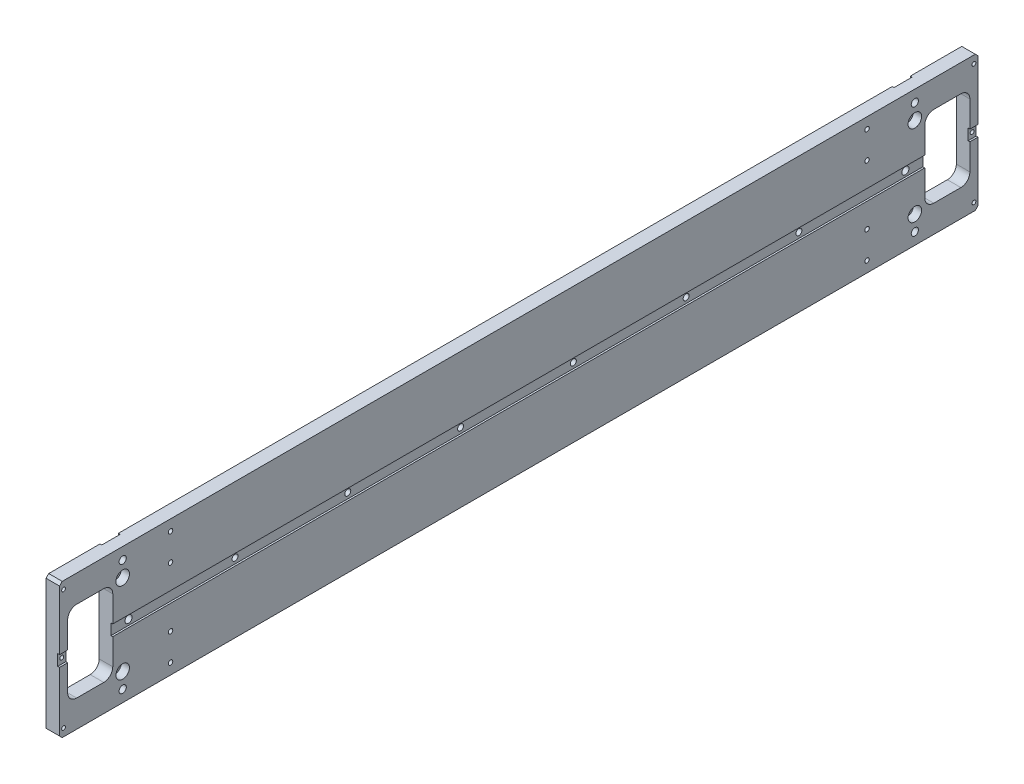
from build123d import *

# Parameters (mm, degrees)
SKETCH_1_W                  = 1018
SKETCH_1_H                  = 150
EXTRUDE_1_DEPTH             = 15
SKETCH_2_W                  = 1412.201465812
SKETCH_2_H                  = 12.2
CUT_EXTRUDE_1_DEPTH         = 2
SKETCH_15_W                 = 20.2
SKETCH_15_H                 = 532.053707348
SKETCH_15_H_2               = 612.26589084
CUT_EXTRUDE_4_DEPTH         = 2
CHAMFER_1_SIZE              = 3
SKETCH_24_W                 = 50
SKETCH_24_H                 = 90
CUT_EXTRUDE_5_DEPTH         = 515.714483962
FILLET_2_R                  = 10
FILLET_2_OF_MIRROR_1_R      = 10
HOLE_WIZARD_9_D             = 9
HOLE_WIZARD_9_CBORE_D       = 15
HOLE_WIZARD_9_CBORE_DEPTH   = 9
MM_2_AT_2_COUNT             = 2
MM_2_AT_2_PITCH             = 124
HOLE_WIZARD_M6_1_D          = 5
HOLE_WIZARD_9_2_D           = 6.6
HOLE_WIZARD_9_2_CBORE_D     = 11
HOLE_WIZARD_9_2_CBORE_DEPTH = 6.8
MM_3_D                      = 8
HOLE_WIZARD_0_D             = 4.3
HOLE_WIZARD_0_CBORE_D       = 8
HOLE_WIZARD_0_CBORE_DEPTH   = 5


with BuildPart() as part:
    # 草图1 → 凸台-拉伸1 (new body)
    with BuildSketch(Plane(origin=(0, 0, 0), x_dir=(0, 0, -1), z_dir=(1, 0, 0))):
        Rectangle(SKETCH_1_W, SKETCH_1_H)
    extrude(amount=EXTRUDE_1_DEPTH)

    # 草图2 → 切除-拉伸1 (cut)
    with BuildSketch(Plane(origin=(15, 0, 0), x_dir=(0, 0, -1), z_dir=(1, 0, 0))):
        Rectangle(SKETCH_2_W, SKETCH_2_H)
    extrude(amount=-CUT_EXTRUDE_1_DEPTH, mode=Mode.SUBTRACT)

    # 草图15 → 切除-拉伸4 (cut)
    with BuildSketch(Plane.ZY):
        with Locations((-439, -14.180103386)):
            Rectangle(SKETCH_15_W, SKETCH_15_H)
        with Locations((439, -22.190357802)):
            Rectangle(SKETCH_15_W, SKETCH_15_H_2)
    extrude(amount=-CUT_EXTRUDE_4_DEPTH, mode=Mode.SUBTRACT)

    # 倒角1
    chamfer_1_edges = [part.edges().sort_by_distance(p)[0] for p in [
        (7.5, 75, 509),
        (7.5, 75, -509),
        (7.5, -75, -509),
        (7.5, -75, 509),
    ]]
    chamfer(chamfer_1_edges, length=CHAMFER_1_SIZE)

    # 草图24 → 切除-拉伸5 (cut, through all)
    with BuildSketch(Plane(origin=(15, 0, 0), x_dir=(0, 0, -1), z_dir=(1, 0, 0))):
        with Locations((-475, 0)):
            Rectangle(SKETCH_24_W, SKETCH_24_H)
    cut_extrude_5 = extrude(amount=-CUT_EXTRUDE_5_DEPTH, mode=Mode.SUBTRACT)

    # 圆角2
    fillet_2_edges = [part.edges().sort_by_distance(p)[0] for p in [
        (7.5, 45, 450),
        (7.5, -45, 500),
        (7.5, -45, 450),
        (7.5, 45, 500),
    ]]
    fillet(fillet_2_edges, radius=FILLET_2_R)

    # 镜向1: 切除-拉伸5 across plane
    add(cut_extrude_5.mirror(Plane.XY), mode=Mode.SUBTRACT)

    # 圆角2 of 镜向1
    fillet_2_of_mirror_1_edges = [part.edges().sort_by_distance(p)[0] for p in [
        (7.5, 45, -450),
        (7.5, -45, -500),
        (7.5, -45, -450),
        (7.5, 45, -500),
    ]]
    fillet(fillet_2_of_mirror_1_edges, radius=FILLET_2_OF_MIRROR_1_R)

    # Hole Wizard 9 (through all)
    with Locations(Plane(origin=(15, 0, 0), x_dir=(0, 0, -1), z_dir=(1, 0, 0))):
        with Locations((439, 45), (439, -45)):
            hole_wizard_9 = CounterBoreHole(HOLE_WIZARD_9_D / 2, HOLE_WIZARD_9_CBORE_D / 2, HOLE_WIZARD_9_CBORE_DEPTH)

    # 草图34 → 大小mm 暗销孔2 (revolve, cut)
    with BuildSketch(Plane(origin=(15, 62, -439), x_dir=(0, 0, -1), z_dir=(0, 1, 0))):
        Polygon((0, 0), (0, 17.403442476), (4, 15), (4, 0), align=None)
    mm_2 = revolve(axis=Axis((21.35, 62, -439), (-1, 0, 0)), mode=Mode.SUBTRACT)

    # 大小mm 暗销孔2 at 2: 大小mm 暗销孔2 ×2
    with Locations(*[(0, -i * MM_2_AT_2_PITCH, 0) for i in range(1, MM_2_AT_2_COUNT)]):
        add(mm_2, mode=Mode.SUBTRACT)

    # M6 螺纹孔1 (through all)
    with Locations(Plane.ZY):
        with Locations((-386, 63), (-386, 33), (-386, -33), (-386, -63)):
            hole_wizard_m6_1 = Hole(HOLE_WIZARD_M6_1_D / 2)

    # Hole Wizard 9 2 (through all)
    with Locations(Plane.ZY):
        with Locations((-312.5, 0), (-187.5, 0), (-62.5, 0), (62.5, 0), (187.5, 0), (312.5, 0)):
            CounterBoreHole(HOLE_WIZARD_9_2_D / 2, HOLE_WIZARD_9_2_CBORE_D / 2, HOLE_WIZARD_9_2_CBORE_DEPTH)

    # 大小mm 暗销孔3 (through all)
    with Locations(Plane.ZY):
        with Locations((430.5, 0), (-430.5, 0)):
            mm_3 = Hole(MM_3_D / 2)

    # 打孔尺寸(%根据)内六角圆柱头螺钉的类型0 (through all)
    with Locations(Plane.ZY):
        with Locations((-504.5, 66.5), (-504.5, 0), (-504.5, -66.5)):
            hole_wizard_0 = CounterBoreHole(HOLE_WIZARD_0_D / 2, HOLE_WIZARD_0_CBORE_D / 2, HOLE_WIZARD_0_CBORE_DEPTH)

    # 镜向2: Hole Wizard 9, 大小mm 暗销孔2, M6 螺纹孔1, 大小mm 暗销孔3, 打孔尺寸(%根据)内六角圆柱头螺钉的类型0 across plane
    add(hole_wizard_9.mirror(Plane.XY), mode=Mode.SUBTRACT)
    add(mm_2.mirror(Plane.XY), mode=Mode.SUBTRACT)
    add(hole_wizard_m6_1.mirror(Plane.XY), mode=Mode.SUBTRACT)
    add(mm_3.mirror(Plane.XY), mode=Mode.SUBTRACT)
    add(hole_wizard_0.mirror(Plane.XY), mode=Mode.SUBTRACT)

    # 镜向2 copy 1 sketch → 镜向2 copy 1 (revolve, cut)
    with BuildSketch(Plane(origin=(15, -62, 439), x_dir=(0, 0, 1), z_dir=(0, 1, 0))):
        Polygon((0, 0), (0, -17.403442476), (4, -15), (4, 0), align=None)
    revolve(axis=Axis((21.35, -62, 439), (1, 0, 0)), mode=Mode.SUBTRACT)


solid = part.part
